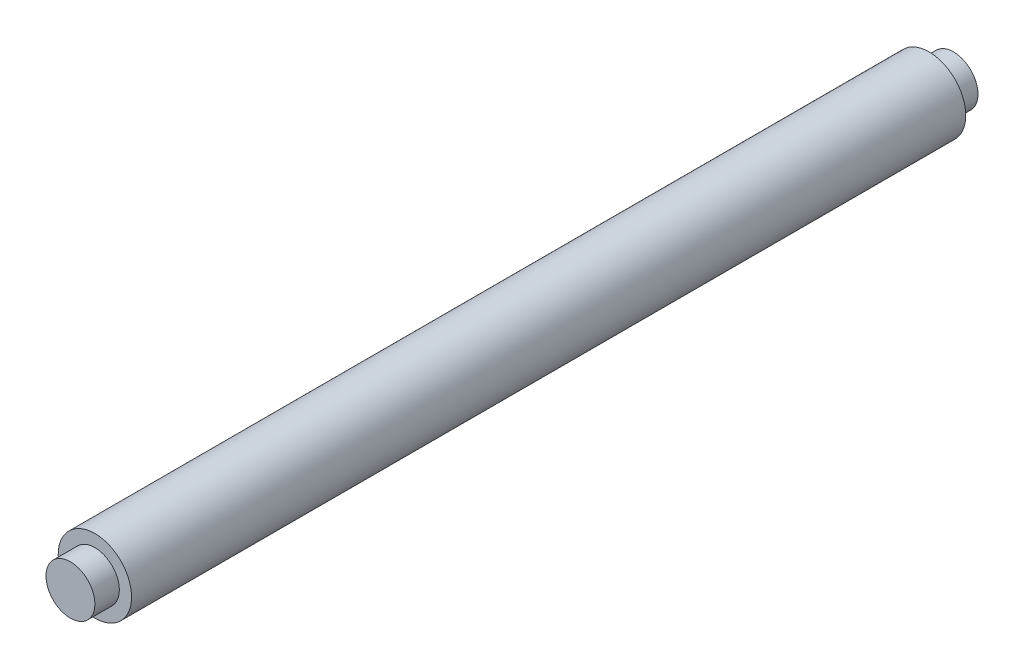
from build123d import *

# Parameters (mm, degrees)
SKETCH_1_R      = 15
EXTRUDE_1_DEPTH = 170.5
SKETCH_2_R      = 10
EXTRUDE_2_DEPTH = 10


with BuildPart() as part:
    # 草图1 → 凸台-拉伸1 (new, symmetric)
    with BuildSketch(Plane.XY):
        with Locations(Location((0, 0, 0), (0, 0, 180))):
            Circle(SKETCH_1_R)
    extrude(amount=EXTRUDE_1_DEPTH, both=True)

    # 草图2 → 凸台-拉伸2 (add)
    with BuildSketch(Plane.XY.offset(170.5)):
        Circle(SKETCH_2_R)
    extrude_2 = extrude(amount=EXTRUDE_2_DEPTH)

    # 镜向1: 凸台-拉伸2 across plane
    add(extrude_2.mirror(Plane.XY))


solid = part.part
